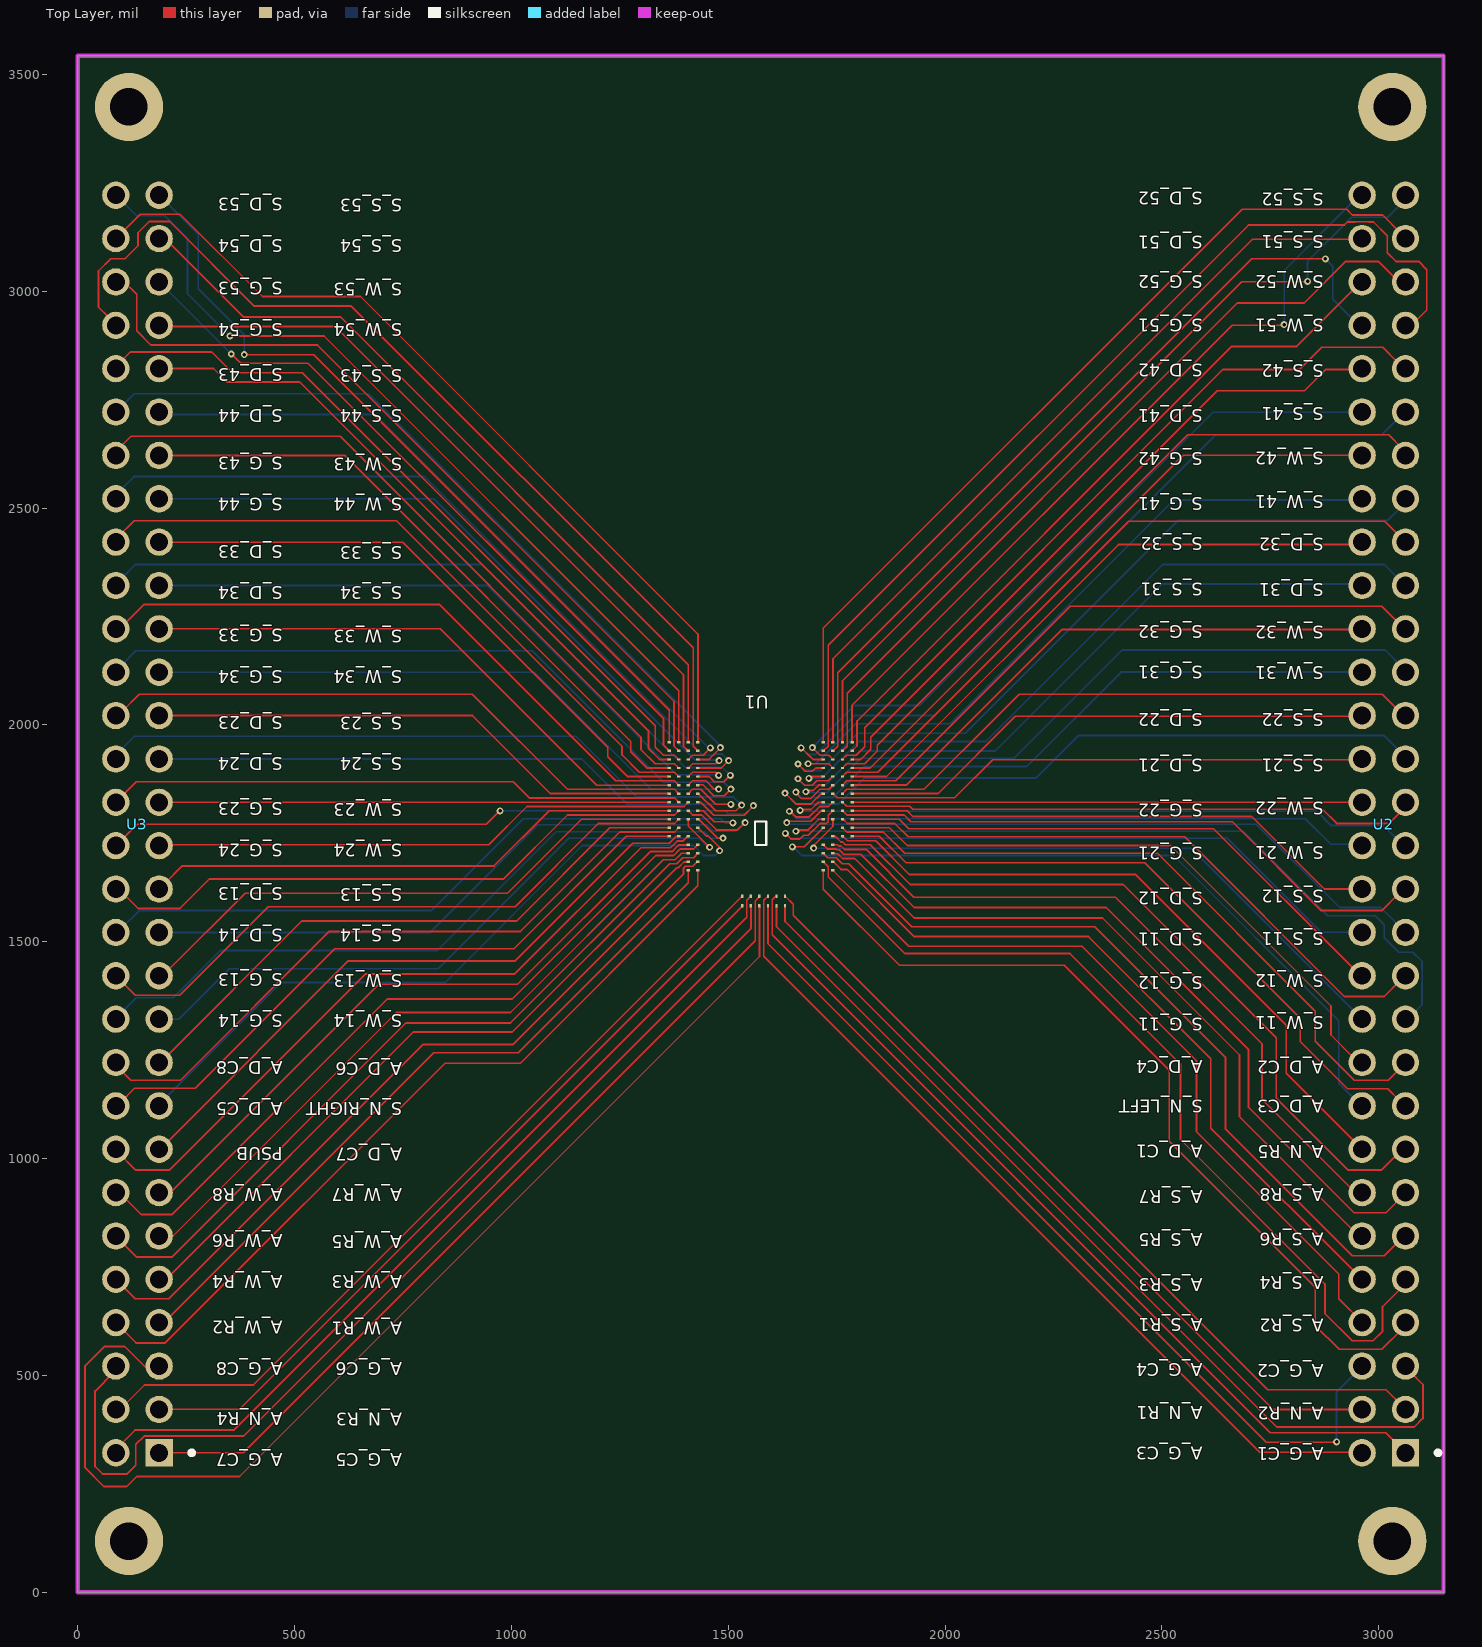
[diagram p0: Top Layer view]
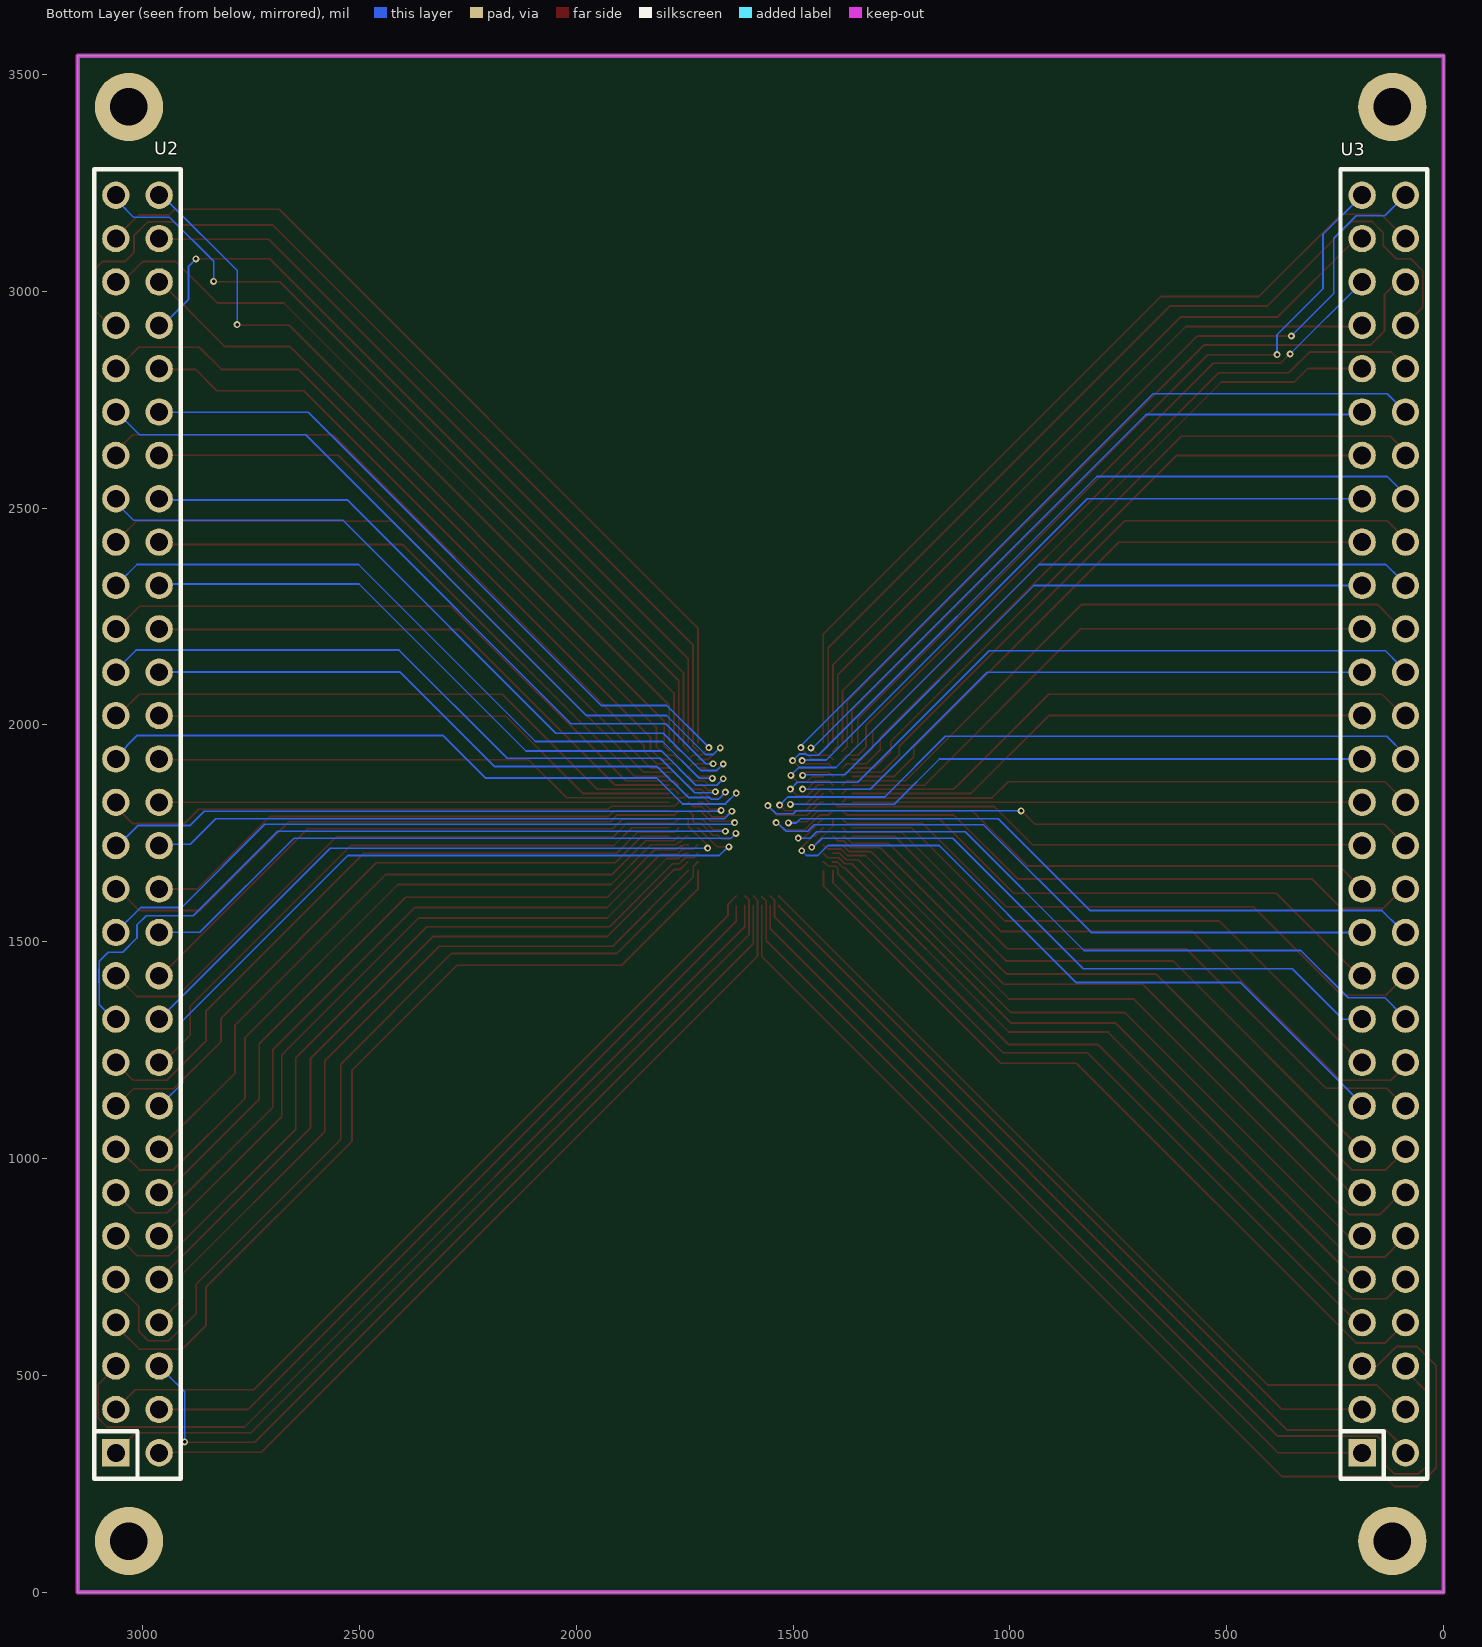
[diagram p1: Bottom Layer view, seen from below]
# Altium PCB MISC82787.pcbdoc
Units mil, origin at the board's own origin, x right, y up, seen from the top; angles counter-clockwise.
Board outline 3149.61 x 3543.31 mil, 2 copper layers (Top Layer, Bottom Layer); 3 components, 120 nets, 244 pads, 40 vias.

## Layer stack, top to bottom (the 12.6 mil dielectric is the usual default, probably not edited)
Top Layer: signal copper 1.4
Dielectric: dielectric 12.6, FR-4, Dk 4.8
Bottom Layer: signal copper 1.4

## Board outline
0,0 3149.61,0 3149.61,3543.31 0,3543.31

## Design rules (kind name [scope] priority, off if disabled: settings)
Clearance [All] p1: gap=5
MinimumSolderMaskSliver [All] p1: minsoldermaskwidth=0
PolygonConnect [All] p1: connectstyle=Relief reliefconductorwidth=10 reliefentries=4 polygonreliefangle="90 Angle"
RoutingVias [All] p1: holewidth=8 width=16 viastyle="Through Hole" minholewidth=8 minwidth=16 maxholewidth=8 maxwidth=16
SilkToSilkClearance [All] p1: silktosilkclearance=0
SilkscreenOverComponentPads [IsPad] p1: minsilkscreentomaskgap=0
SolderMaskExpansion [All] p1: expansion=4
Width [All] p1: maxlimit=4 minlimit=4 preferedwidth=4
25 further rules are at their usual default settings.

## Components (designator, comment, footprint, x,y, rotation, side; value= is the part's Value field where it differs from the comment)
U1 "" XP 1574.8,1771.65 r180 top locked
U2 "P125-1230A0BS116A1" HDR-TH_60P-P2.54-V-M-R2-C30-S2.54-1 3011.81,1771.65 r90 top locked
U3 "P125-1230A0BS116A1" HDR-TH_60P-P2.54-V-M-R2-C30-S2.54-1 137.8,1771.65 r90 top locked

## Footprints (in the part's own frame and the unit in brackets; to place one, negate y for a bottom-side part, rotate by r counter-clockwise, add the part's x,y. Pads: shape width x height; smd on the part's side, far side on the other; paste and mask are expansions set on the pad)
HDR-TH_60P-P2.54-V-M-R2-C30-S2.54-1 [mm]
  rect 1.6x1.6 hole 1.05: 1(-36.83,-1.27)
  round 1.6 hole 1.05: 2(-36.83,1.27) 3(-34.29,-1.27) 4(-34.29,1.27) 5(-31.75,-1.27) 6(-31.75,1.27) 7(-29.21,-1.27) 8(-29.21,1.27) 9(-26.67,-1.27) 10(-26.67,1.27) 11(-24.13,-1.27) 12(-24.13,1.27) 13(-21.59,-1.27) 14(-21.59,1.27) 15(-19.05,-1.27) 16(-19.05,1.27) 17(-16.51,-1.27) 18(-16.51,1.27) 19(-13.97,-1.27) 20(-13.97,1.27) 21(-11.43,-1.27) 22(-11.43,1.27) 23(-8.89,-1.27) 24(-8.89,1.27) 25(-6.35,-1.27) 26(-6.35,1.27) 27(-3.81,-1.27) 28(-3.81,1.27) 29(-1.27,-1.27) 30(-1.27,1.27) 31(1.27,-1.27) 32(1.27,1.27) 33(3.81,-1.27) 34(3.81,1.27) 35(6.35,-1.27) 36(6.35,1.27) 37(8.89,-1.27) 38(8.89,1.27) 39(11.43,-1.27) 40(11.43,1.27) 41(13.97,-1.27) 42(13.97,1.27) 43(16.51,-1.27) 44(16.51,1.27) 45(19.05,-1.27) 46(19.05,1.27) 47(21.59,-1.27) 48(21.59,1.27) 49(24.13,-1.27) 50(24.13,1.27) 51(26.67,-1.27) 52(26.67,1.27) 53(29.21,-1.27) 54(29.21,1.27) 55(31.75,-1.27) 56(31.75,1.27) 57(34.29,-1.27) 58(34.29,1.27) 59(36.83,-1.27) 60(36.83,1.27)
  silkscreen extent -36.96,-3.3 -36.7,-3.05
XP [mm]
  rect 0.14x0.2 smd: 1(-0.93,4.22) 2(-0.43,4.22) 3(-1.43,4.22) 4(-1.43,4.78) 5(-0.93,4.78) 6(-0.43,4.78) 115(0.07,4.78) 116(0.57,4.78) 117(1.07,4.78) 118(1.07,4.22) 119(0.07,4.22) 120(0.57,4.22)
  rect 0.2x0.14 smd: 7(-3.675,2.72) 8(-4.235,2.72) 9(-3.675,2.22) 10(-4.235,2.22) 11(-3.675,1.72) 12(-4.235,1.72) 13(-3.675,1.22) 14(-4.235,1.22) 15(-4.235,0.72) 16(-4.795,0.72) 17(-5.355,0.72) 18(-3.675,0.22) 19(-4.795,0.22) 20(-5.355,0.22) 21(-3.675,-0.28) 22(-4.235,-0.28) 23(-4.795,-0.28) 24(-5.355,-0.28) 25(-3.675,-0.78) 26(-4.235,-0.78) 27(-4.795,-0.78) 28(-5.355,-0.78) 29(-3.675,-1.28) 30(-4.235,-1.28) 31(-4.795,-1.28) 32(-5.355,-1.28) 33(-3.675,-1.78) 34(-4.235,-1.78) 35(-4.795,-1.78) 36(-5.355,-1.78) 37(-3.675,-2.28) 38(-4.235,-2.28) 39(-4.795,-2.28) 40(-5.355,-2.28) 41(-3.675,-2.78) 42(-4.235,-2.78) 43(-4.795,-2.78) 44(-5.355,-2.78) 45(-3.675,-3.28) 46(-4.235,-3.28) 47(-4.795,-3.28) 48(-5.355,-3.28) 49(-3.675,-3.78) 50(-4.235,-3.78) 51(-4.795,-3.78) 52(-5.355,-3.78) 53(-3.675,-4.28) 54(-4.235,-4.28) 55(-4.795,-4.28) 56(-5.355,-4.28) 57(-3.675,-4.78) 58(-4.235,-4.78) 59(-4.795,-4.78) 60(-5.355,-4.78) 61(5.355,-4.78) 62(4.795,-4.78) 63(4.235,-4.78) 64(3.675,-4.78) 65(5.355,-4.28) 66(4.795,-4.28) 67(4.235,-4.28) 68(3.675,-4.28) 69(5.355,-3.78) 70(4.795,-3.78) 71(4.235,-3.78) 72(3.675,-3.78) 73(5.355,-3.28) 74(4.795,-3.28) 75(4.235,-3.28) 76(3.675,-3.28) 77(5.355,-2.78) 78(4.795,-2.78) 79(4.235,-2.78) 80(3.675,-2.78) 81(5.355,-2.28) 82(4.795,-2.28) 83(4.235,-2.28) 84(3.675,-2.28) 85(5.355,-1.78) 86(4.795,-1.78) 87(4.235,-1.78) 88(3.675,-1.78) 89(5.355,-1.28) 90(4.795,-1.28) 91(4.235,-1.28) 92(3.675,-1.28) 93(5.355,-0.78) 94(4.795,-0.78) 95(4.235,-0.78) 96(3.675,-0.78) 97(5.355,-0.28) 98(4.795,-0.28) 99(4.235,-0.28) 100(3.675,-0.28) 101(5.355,0.22) 102(4.795,0.22) 103(3.675,0.22) 104(5.355,0.72) 105(4.795,0.72) 106(4.235,0.72) 107(4.235,1.22) 108(3.675,1.22) 109(4.235,1.72) 110(3.675,1.72) 111(4.235,2.22) 112(3.675,2.22) 113(4.235,2.72) 114(3.675,2.72)
  silkscreen extent -0.32,-0.14 0.33,1.23

## Part data
U1: library part Chip3Array

## Free pads (board coordinates)
  round 157.48 hole 86.61: 0(118.11,118.11) 0(118.11,3425.2) 0(3031.5,118.11) 0(3031.5,3425.2)

## Via types
v1: diameter 16, hole 8, Top Layer to Bottom Layer, 40 vias

## Nets (pads, with @x,y where several pads share a name; then routed paths per layer and width w, separated by ;. In a path a pad name is that pad's centre, name@x,y a point inside that pad or via, vN(x,y) a via of type N, cw(c..) or ccw(c..) an arc to the next point about the centre after c; other vN are vias at no path point)
A_D_C1: U1.16 U2.16 | length 1547.7
  Top Layer w4: U1.16 U1.16@1765.44,1741.44 ; U1.16@1766,1742 1775,1733 1840,1733 1918,1655 2440,1655 2787,1308 2787,1197 U2.16@2952,1032
A_D_C2: U1.19 U2.19 | length 1573.8
  Top Layer w4: U1.19 1773.34,1753.24 1857.76,1753.24 1907,1704 2490,1704 2854,1340 2854,1271 2944,1181 3022,1181 U2.19@3046,1205
A_D_C3: U1.17 U2.17 | length 1546.4
  Top Layer w4: U1.17 1848.69,1743.31 1910,1682 2461,1682 2819,1324 2819,1270 2928,1161 3021,1161 U2.17@3048,1134
A_D_C4: U1.20 U2.20 | length 1415.1
  Top Layer w4: U1.20 1872.01,1762.99 1913,1722 2520,1722 2890,1352 2890,1285 U2.20@2942,1233
A_D_C5: U1.104 U3.18 | length 1520.4
  Top Layer w4: U3.18@98,1129 131,1162 271,1162 593,1484 1006,1484 1265.31,1743.31 U1.104
A_D_C6: U1.101 U3.19 | length 1378.7
  Top Layer w4: U3.19@204,1235 517,1548 1012,1548 1226.99,1762.99 U1.101
A_D_C7: U1.105 U3.15 | length 1473.6
  Top Layer w4: U3.15@205,1037 624,1456 1009,1456 1280,1727 1364,1727 1364.26,1727 1380.57,1743.31 U1.105
A_D_C8: U1.102 U3.20 | length 1546.1
  Top Layer w4: U3.20@93,1210 122,1181 237,1181 580,1524 1021,1524 1250.06,1753.06 1376.09,1753.06 U1.102
A_G_C1: U1.1 U2.1 | length 2016
  Top Layer w4: U1.1@1610,1605 1601.66,1596.66 1601.66,1516.34 2750,368 3016,368 U2.1@3039,345 ; U1.1@1610.45,1604.55 U1.1
A_G_C2: U1.5 U2.5 | length 2143.2
  Top Layer w4: U1.5 1611.42,1534.58 2765,381 3082,381 3102,401 3102,479 U2.5@3074,507
A_G_C3: U1.2 U2.2 | length 1978.4
  Top Layer w4: U1.2 1581.98,1595.76 1581.98,1467.02 2726,323 U2.2@2944,323
A_G_C4: U1.6 U2.6 | length 2050.9
  Top Layer w4: U1.6 1591.73,1495.27 2741,346 2903,346 v1(2903,347)
  Bottom Layer w4: v1(2903,347) 2903,462 U2.6@2945,504
A_G_C5: U1.119 U3.1 | length 1969.3
  Top Layer w4: U3.1 381.65,321.65 1562.12,1502.12 1562.12,1594.12 U1.119@1572,1604
A_G_C6: U1.115 U3.5 | length 2634.6
  Top Layer w4: U3.5@182,520 155,520 108,567 62,567 17,522 17,287 60,244 113,244 136,267 373,267 1572.05,1466.05 U1.115
A_G_C7: U1.120 U3.2 | length 1995.8
  Top Layer w4: U3.2@102,344 132,374 360,374 1542.61,1556.61 1542.61,1595.76 U1.120
A_G_C8: U1.116 U3.6 | length 2356.3
  Top Layer w4: U3.6@83,507 40,464 40,290 57,273 114,273 134,293 134,341 153.15,360.15 382.15,360.15 1552.36,1530.36 U1.116
A_N_R1: U1.4 U2.4 | length 1832.9
  Top Layer w4: U1.4@1631,1583 1631,1547 2756.35,421.65 U2.4
A_N_R2: U1.3 U2.3 | length 1924.8
  Top Layer w4: U1.3 1649.81,1586.81 1649.81,1561.19 2744,467 3017,467 U2.3@3054,430
A_N_R3: U1.117 U3.3 | length 1819.8
  Top Layer w4: U3.3@195,422 373,422 1532.68,1581.68 U1.117
A_N_R4: U1.118 U3.4 | length 1909.3
  Top Layer w4: U3.4@109,433 154,478 405.17,478 U1.118
A_N_R5: U1.15 U2.15 | length 1715.6
  Top Layer w4: U1.15 1746.69,1743.31 1759.99,1730.01 1763.9,1730.01 1769.91,1724 1828,1724 1920,1632 2411,1632 2764,1279 2764,1139 2929,974 3007,974 U2.15@3042,1009
A_S_R1: U1.8 U2.8 | length 1784.2
  Top Layer w4: U1.8 1916.1,1490 2316,1490 2580,1226 2580,1062 2908,734 2908,677 U2.8@2964,621
A_S_R2: U1.7 U2.7 | length 1985.6
  Top Layer w4: U1.7 1719.49,1621.51 1895,1446 2275,1446 2517,1204 2517,1040 2854,703 2854,615 2908.85,560.15 3007.15,560.15 U2.7@3055,608
A_S_R3: U1.10 U2.10 | length 1710.9
  Top Layer w4: U1.10@1743,1684 1760,1667 1774,1667 1929,1512 2331,1512 2613,1230 2613,1070.46 U2.10
A_S_R4: U1.9 U2.9 | length 2032.3
  Top Layer w4: U1.9 1730.43,1673.32 1730.43,1649.57 1907,1473 2288,1473 2543,1218 2543,1044 2876,711 2876,643 2939,580 2987,580 3009,602 3009,659 U2.9@3054,704
A_S_R5: U1.12 U2.12 | length 1647.9
  Top Layer w4: U1.12 U1.12@1743.06,1703.94 ; U1.12@1742,1704 1746,1704 1746.99,1703.01 1752.72,1703.01 1763.73,1692 1792,1692 1929,1555 2363,1555 2679,1239 2679,1097 U2.12@2944,832
A_S_R6: U1.11 U2.11 | length 1817
  Top Layer w4: U1.11 1729.42,1694.01 1748.99,1694.01 1763,1680 1778,1680 1923,1535 2345,1535 2647,1233 2647,1068 2939,776 3013,776 U2.11@3043,806
A_S_R7: U1.14 U2.14 | length 1595.4
  Top Layer w4: U1.14 U1.14@1742.08,1723.08 ; U1.14@1743,1724 1752,1724 1754.99,1721.01 1760.18,1721.01 1768.18,1713 1818,1713 1928,1603 2393,1603 2731,1265 2731,1137 U2.14@2935,933
A_S_R8: U1.13 U2.13 | length 1773.6
  Top Layer w4: U1.13 1729.24,1713.87 1748.86,1713.87 1749.73,1713 1750.72,1712.01 1756.45,1712.01 1766.46,1702 1806,1702 1929,1579 2372,1579 2700,1251 2700,1118 2943,875 3017,875 U2.13@3050,908
A_W_R1: U1.113 U3.7 | length 1642.1
  Top Layer w4: U3.7@210,633 821,1244 1016,1244 1408.07,1636.07 U1.113
A_W_R2: U1.114 U3.8 | length 1833.1
  Top Layer w4: U3.8 134.45,575 202,575 847,1220 1021,1220 1430,1629 U1.114@1430,1664
A_W_R3: U1.111 U3.9 | length 1592.2
  Top Layer w4: U3.9@212,730 774,1292 1002,1292 1381,1671 1383,1671 1385,1671 1398,1684 1408.07,1684 U1.111@1409,1684
A_W_R4: U1.112 U3.10 | length 1785.2
  Top Layer w4: U3.10 132.45,677 210,677 796,1263 1003,1263 1397.13,1657.13 1397.13,1670.22 1401.23,1674.32 1415.1,1674.32 1418.32,1674.32 U1.112@1429,1685 ; U1.112@1429.93,1684.07 U1.112
A_W_R5: U1.109 U3.11 | length 1585.8
  Top Layer w4: U3.11 219.65,821.65 735,1337 998,1337 1350,1689 1374.27,1689 1377.27,1689 1390.22,1701.95 ; 1390.17,1702 1392.11,1703.94 U1.109 U1.109@1408,1703.94
A_W_R6: U1.110 U3.12 | length 1737.7
  Top Layer w4: U3.12@95,814 136,773 217,773 757,1313 998,1313 1365,1680 1381,1680 1395.01,1694.01 1420.19,1694.01 U1.110
A_W_R7: U1.107 U3.13 | length 1554.1
  Top Layer w4: U3.13 213.65,921.65 694,1402 1014,1402 1320,1708 1370.72,1708 1380.72,1718 1385.58,1722.87 1385.72,1723 1387.73,1723 1403,1723 U1.107@1408,1723 ; U1.107@1408,1723.62 U1.107 ; U1.107@1408.07,1723 U1.107@1410,1723
A_W_R8: U1.108 U3.14 | length 1689.4
  Top Layer w4: U3.14@110,908 147,871 217,871 714,1368 1002,1368 1333,1699 1374.45,1699 1388.45,1713 1389.31,1713.87 ; 1389.45,1714 1389.31,1713.87 ; U1.108@1428.75,1722.25 U1.108 ; U1.108@1429,1723 1420,1714 1415.04,1714 1415.04,1713.87 1407,1713.87 1389.31,1713.87
PSUB: U1.106 U3.16 | length 1648.6
  Top Layer w4: U3.16@94,1013 133,974 212,974 664,1426 1008,1426 1299,1717 1366.99,1717 1381.99,1732 1382.62,1732.62 1396.62,1732.62 U1.106@1407,1743 ; U1.106@1407.5,1742.5 U1.106@1408,1743 ; U1.106@1407.88,1743.12 U1.106
S_D_11: U1.26 U2.26 | length 1568.8
  Top Layer w4: v1(1632,1750) 1645,1737 1665,1737 1674,1746 1685,1746 1711.92,1772.92 1726.32,1772.92 1730.6,1777.2 1730.6,1791.43 U1.26
  Bottom Layer w4: v1(1632,1750) 1643,1739 2651,1739 2868,1522 U2.26@2956,1522
S_D_12: U1.28 U2.28 | length 1251
  Top Layer w4: U1.28 1912.64,1802.36 1926,1789 2707,1789 2874.35,1621.65 U2.28
S_D_13: U1.94 U3.28 | length 1392.7
  Top Layer w4: U3.28@102,1614 139,1577 236,1577 304,1645 982,1645 1129.43,1792.43 1376.09,1792.43 U1.94
S_D_14: U1.96 U3.26 | length 1610.2
  Top Layer w4: U1.96 1442.64,1802.36 1468,1777 1508,1777 v1(1511,1774)
  Bottom Layer w4: U3.26@102,1532 142,1572 815,1572 1027,1784 1483,1784 1493,1774 v1(1511,1774)
S_D_21: U1.34 U2.34 | length 1244
  Top Layer w4: U1.34 1751.29,1831.98 2021.98,1831.98 2110,1920 U2.34@2945,1920
S_D_22: U1.36 U2.36 | length 1238.2
  Top Layer w4: U1.36 1983.73,1841.73 2162,2020 U2.36@2950,2020
S_D_23: U1.86 U3.36 | length 1395.6
  Top Layer w4: U3.36@102,2031 142,2071 910,2071 1129.34,1851.66 1376.09,1851.66 U1.86
S_D_24: U1.88 U3.34 | length 1646.6
  Top Layer w4: U1.88 1431.27,1841.73 1471,1802 1518,1802 v1(1531,1815)
  Bottom Layer w4: U3.34@90,1933 131,1974 1149,1974 1289,1834 1512,1834 v1(1531,1815)
S_D_31: U1.41 U2.41 | length 1625.8
  Top Layer w4: v1(1686,1877) 1690.1,1881.1 U1.41
  Bottom Layer w4: v1(1686,1877) 1716,1877 1801,1962 2094,1962 2502,2370 3013,2370 U2.41@3055,2328
S_D_32: U1.43 U2.43 | length 1543.8
  Top Layer w4: U1.43 1773.48,1891 1845,1891 2424,2470 3014,2470 U2.43@3049,2435
S_D_33: U1.78 U3.44 | length 1564.4
  Top Layer w4: U3.44@93,2434 130,2471 735,2471 1255,1951 1255,1931 1295.14,1890.86 1376.27,1890.86 U1.78
S_D_34: U1.80 U3.42 | length 1707.5
  Top Layer w4: U1.80 1455.9,1881.1 1468,1869 1490,1869 v1(1505,1884)
  Bottom Layer w4: U3.42@99,2336 133,2370 933,2370 1401,1902 1487,1902 v1(1505,1884)
S_D_41: U1.50 U2.50 | length 1631.1
  Top Layer w4: v1(1694,1948) 1711.77,1930.23 1731.78,1930.23 U1.50
  Bottom Layer w4: v1(1694,1948) 1705,1959 1791,2045 1942,2045 2618,2721 U2.50@2946,2721
S_D_42: U1.52 U2.52 | length 1561.4
  Top Layer w4: U1.52 1805.47,1920.47 1829,1944 1829,1972 2628,2771 2829,2771 2878,2820 U2.52@2958,2820
S_D_43: U1.70 U3.52 | length 1720.4
  Top Layer w4: U3.52@96,2833 96,2835 121.15,2860.15 308.85,2860.15 357,2812 518,2812 1332,1998 1332,1949 1350.77,1930.23 1376.27,1930.23 U1.70
S_D_44: U1.72 U3.50 | length 1814.8
  Top Layer w4: U1.72 1455.47,1920.47 1482,1947 v1(1482,1948)
  Bottom Layer w4: U3.50 130.14,2764 670,2764 v1@1484,1950
S_D_51: U1.58 U2.58 | length 1810.9
  Top Layer w4: U1.58 1741.54,2152.54 2709,3120 U2.58@2959,3120
S_D_52: U1.60 U2.60 | length 1800.7
  Top Layer w4: U1.60 1785.63,2045.63 2662,2922 v1@2781,2922 ; v1@2782,2922 v1@2781,2922 ; v1(2782,2923) v1@2781,2922
  Bottom Layer w4: v1(2782,2923) 2782,3048 U2.60@2944,3210
S_D_53: U1.62 U3.60 | length 1965.1
  Top Layer w4: v1(351,2897) 568,2897 1386.02,2078.98 U1.62
  Bottom Layer w4: U3.60 135.45,3174 201,3174 253,3122 253,2995 v1(351,2897)
S_D_54: U1.64 U3.58 | length 2016.7
  Top Layer w4: U3.58 144.14,3178 236,3178 426,2988 652,2988 1430.12,2209.88 U1.64
S_G_11: U1.22 U2.22 | length 1509.7
  Top Layer w4: v1@1696,1716 v1(1697,1716) ; v1@1696,1721 1741.54,1766.54 U1.22
  Bottom Layer w4: v1(1697,1716) 2567.46,1716 U2.22
S_G_12: U1.24 U2.24 | length 1306.2
  Top Layer w4: U1.24 1894.32,1782.68 1916,1761 2619,1761 U2.24@2947,1433
S_G_13: U1.98 U3.24 | length 1473.4
  Top Layer w4: U3.24@96,1414 133,1377 235,1377 439,1581 1009,1581 1200.75,1772.75 1376.09,1772.75 U1.98
S_G_14: U1.100 U3.22 | length 1649
  Top Layer w4: U1.100 1432.32,1782.68 1476,1739 v1(1488,1739)
  Bottom Layer w4: U3.22@96,1332 135,1371 220,1371 329,1480 829,1480 1103,1754 1445,1754 1460,1739 v1(1488,1739)
S_G_21: U1.30 U2.30 | length 1459.8
  Top Layer w4: v1(1641,1801) v1@1644,1798 ; v1@1645,1799 1656,1788 1687,1788 1711.12,1812.12 1726.44,1812.12 1731.12,1812.12 U1.30@1741,1822 ; U1.30@1741.24,1821.76 U1.30
  Bottom Layer w4: v1@1640,1801 v1(1641,1801) 1658,1784 2831,1784 2890,1725 U2.30@2949,1725
S_G_22: U1.32 U2.32 | length 1158.3
  Top Layer w4: U1.32 U2.32@2943.95,1822.05
S_G_23: U1.90 U3.32 | length 1312.9
  Top Layer w4: U3.32@105,1839 135,1869 1004,1869 1041.2,1831.8 1376.27,1831.8 U1.90
S_G_24: U1.92 U3.30 | length 1655.9
  Top Layer w4: U3.30 137.14,1771 942,1771 v1@971,1800 ; U1.92 1436.95,1822.05 1467,1792 1537,1792 v1@1556,1811 ; v1@1555.5,1811.5 v1(1558,1814)
  Bottom Layer w4: v1(974,1802) 1409,1802 1493,1802 1500,1795 1539,1795 v1@1555,1811
S_G_31: U1.38 U2.38 | length 1514.5
  Top Layer w4: v1(1656,1845) v1@1659,1842 ; v1@1658,1841 1668,1831 1691,1831 1711.66,1851.66 1731.66,1851.66 1741.42,1861.42 U1.38
  Bottom Layer w4: v1(1656,1845) 1672,1829 1689,1829 1693,1833 1742,1833 1813,1904 2188,1904 2406,2122 U2.38@2938,2122
S_G_32: U1.40 U2.40 | length 1307.9
  Top Layer w4: U1.40 1910.42,1861.42 2269,2220 U2.40@2945,2220
S_G_33: U1.82 U3.40 | length 1462.1
  Top Layer w4: U3.40@113,2238 153,2278 834,2278 1240.83,1871.17 1376.27,1871.17 U1.82
S_G_34: U1.84 U3.38 | length 1641.8
  Top Layer w4: U1.84 U1.84@1431,1861.42 ; U1.84@1431,1862 1442,1862 1467,1837 1491,1837 v1(1506,1852)
  Bottom Layer w4: U3.38@102,2139 134,2171 1048,2171 1351,1868 1490,1868 v1(1506,1852)
S_G_41: U1.46 U2.46 | length 1580.7
  Top Layer w4: v1(1684.46,1910.54) 1731.78,1910.54 U1.46
  Bottom Layer w4: v1(1684.46,1910.54) 1701.54,1910.54 1794,2003 2012,2003 2528,2519 U2.46@2952,2519
S_G_42: U1.48 U2.48 | length 1459.1
  Top Layer w4: U1.48 1827.79,1900.79 2549,2622 U2.48@2946,2622
S_G_43: U1.74 U3.48 | length 1652.1
  Top Layer w4: U3.48@84,2627 123,2666 605,2666 1299,1972 1299,1943 1331.46,1910.54 1376.27,1910.54 U1.74
S_G_44: U1.76 U3.46 | length 1780.8
  Top Layer w4: U1.76 1483.79,1900.79 v1(1501,1918)
  Bottom Layer w4: U3.46@89,2532 130,2573 799,2573 1442,1930 1468,1930 1471,1933 1485.21,1933 1486.21,1932 1487,1932 v1(1501,1918)
S_G_51: U1.54 U2.54 | length 1869.8
  Top Layer w4: U1.54 1752.65,1951.27 1752.65,2120.65 2707,3075 v1(2877,3075)
  Bottom Layer w4: v1(2877,3075) 2894,3058 2894,2982 U2.54@2940,2936
S_G_52: U1.56 U2.56 | length 1637.8
  Top Layer w4: U1.56 1797,1951.53 1797,2009 2661,2873 2811,2873 U2.56@2947,3009
S_G_53: U1.66 U3.56 | length 1842.2
  Top Layer w4: U3.56@103,3026 136,2993 136,2909 169,2876 553,2876 1374.91,2054.09 1374.91,1951.27 U1.66
S_G_54: U1.68 U3.54 | length 2205.5
  Top Layer w4: U3.54@75,2941 70,2941 48,2963 48,3047 76,3075 109,3075 139,3105 139,3135 165,3161 212,3161 407,2966 631,2966 1419.18,2177.82 1419.18,1951.09 U1.68
S_N_LEFT: U1.18 U2.18 | length 1724.4
  Top Layer w4: v1(1648,1719) 1648,1717 1650,1719 1675.5,1719 U1.18
  Bottom Layer w4: v1(1648,1719) v1@1651,1719 ; v1@1651,1718 1670,1699 2527,1699 2908,1318 2908,1174 U2.18@2952,1130
S_N_RIGHT: U1.103 U3.17 | length 1616.7
  Top Layer w4: U1.103 1449.11,1744 1454,1744 1480,1718 v1(1480,1710)
  Bottom Layer w4: U3.17@197,1135 468,1406 847,1406 1163,1722 1420,1722 1443,1699 1469,1699 v1(1480,1710)
S_S_11: U1.25 U2.25 | length 1624
  Top Layer w4: v1(1635,1775) 1635,1774 v1@1635.5,1774.5 ; v1@1639,1778 1690,1778 1714.36,1802.36 U1.25
  Bottom Layer w4: v1(1635,1775) 1639,1771 2718,1771 2910,1579 3004.46,1579 U2.25
S_S_12: U1.27 U2.27 | length 1391.2
  Top Layer w4: U1.27 1773.34,1792.61 1905.39,1792.61 1921,1777 2663,1777 2868,1572 3007,1572 U2.27@3044,1609
S_S_13: U1.93 U3.27 | length 1233.7
  Top Layer w4: U3.27@200,1634 241,1675 960,1675 1087.36,1802.36 U1.93
S_S_14: U1.95 U3.25 | length 1620.5
  Top Layer w4: U1.95 1417.83,1792.61 1438.39,1792.61 1473,1758 1522,1758 v1(1539,1775)
  Bottom Layer w4: U3.25 812.65,1521.65 1061,1770 1451,1770 1466,1755 1516,1755 v1@1535,1774
S_S_21: U1.33 U2.33 | length 1634.8
  Top Layer w4: v1(1631,1843) 1656,1818 1691,1818 1714.73,1841.73 U1.33
  Bottom Layer w4: v1(1631,1843) 1656,1818 1755,1818 1815,1878 2210,1878 2308,1976 3012,1976 U2.33@3061,1927
S_S_22: U1.35 U2.35 | length 1393.1
  Top Layer w4: U1.35 1773.34,1851.49 1951.49,1851.49 2122.5,2022.5 ; 2124.5,2024.5 2122.5,2022.5 ; U2.35@3044,2035 3008,2071 2171,2071 2122.5,2022.5
S_S_23: U1.85 U3.35 | length 1250.6
  Top Layer w4: U3.35 910.35,2021.65 1090,1842 U1.85@1364,1842
S_S_24: U1.87 U3.33 | length 1473.1
  Top Layer w4: U1.87 1417.83,1851.49 1436.95,1851.49 1441.05,1847.39 1441.05,1846.95 1471,1817 v1(1506,1817)
  Bottom Layer w4: U3.33 1162.35,1921.65 1267,1817 v1@1501,1817
S_S_31: U1.42 U2.42 | length 1579.5
  Top Layer w4: v1(1661,1876) 1676,1861 1694,1861 1704.35,1871.35 1730.35,1871.35 1740.1,1881.1 U1.42
  Bottom Layer w4: v1(1661,1876) 1676,1861 1724,1861 1803,1940 2116,1940 2501,2325 U2.42@2947,2325
S_S_32: U1.44 U2.44 | length 1392.9
  Top Layer w4: U1.44 1865.1,1881.1 2400,2416 U2.44@2957,2416
S_S_33: U1.77 U3.43 | length 1412
  Top Layer w4: U3.43 749.35,2421.65 1222,1949 1222,1927 1268,1881 U1.77@1363,1881
S_S_34: U1.79 U3.41 | length 1546.9
  Top Layer w4: U1.79 1417.83,1890.86 1471.14,1890.86 v1(1478,1884)
  Bottom Layer w4: U3.41 944.35,2321.65 1381,1885 v1@1477,1885
S_S_41: U1.49 U2.49 | length 1770.9
  Top Layer w4: v1(1668,1947) v1@1669,1947 ; v1@1669,1948 v1@1669,1947 ; U1.49 1695.74,1920.47 1690.67,1925.54 1690.46,1925.54 v1@1669,1947
  Bottom Layer w4: v1@1672,1944 1684,1932 1702,1932 1792,2022 1977,2022 2624,2669 3007,2669 U2.49@3051,2713
S_S_42: U1.51 U2.51 | length 1713
  Top Layer w4: U1.51 1773.34,1930.23 1795.23,1930.23 1815,1950 1815,1994 2641,2820 2818,2820 2869,2871 3009,2871 U2.51@3043,2837
S_S_43: U1.69 U3.51 | length 1565.4
  Top Layer w4: U3.51@196,2822 313,2822 344,2791 512,2791 1316,1987 1316,1946 1341.53,1920.47 U1.69
S_S_44: U1.71 U3.49 | length 1634.4
  Top Layer w4: U1.71 1417.83,1930.23 1442.23,1930.23 v1(1459,1947)
  Bottom Layer w4: U3.49@205,2716 686,2716 1455,1947 v1(1459,1947)
S_S_51: U1.57 U2.57 | length 2016.5
  Top Layer w4: U1.57 1719.49,2223.49 2685,3189 2926,3189 2939,3176 3009,3176 U2.57@3050,3135
S_S_52: U1.59 U2.59 | length 1910.3
  Top Layer w4: U1.59 1763.58,2101.58 2684,3022 v1@2831,3022 ; v1@2835,3022 v1(2836,3023)
  Bottom Layer w4: v1(2836,3023) 2836,3069 2938,3171 3021,3171 U2.59@3053,3203
S_S_53: U1.61 U3.59 | length 1842.7
  Top Layer w4: v1(384,2854) 544,2854 1363.98,2034.02 U1.61
  Bottom Layer w4: U3.59 278,3131.45 278,3006 384,2900 v1(384,2854)
S_S_54: U1.63 U3.57 | length 1791.2
  Top Layer w4: U3.57@199,3112 211,3112 382,2941 606,2941 1408.07,2138.93 U1.63
S_W_11: U1.21 U2.21 | length 1790.9
  Top Layer w4: v1(1656,1755) 1659,1758 1684.27,1758 1708.19,1781.92 1708.92,1781.92 1709.68,1782.68 U1.21
  Bottom Layer w4: v1(1656,1755) 2688,1755 2882.85,1560.15 2991.85,1560.15 3013,1539 3013,1509 3046,1476 3079,1476 3100,1455 3100,1437.91 3100.31,1437.6 3100.31,1405.4 3100,1405.4 3100,1355 U2.21@3079,1334
S_W_12: U1.23 U2.23 | length 1470.5
  Top Layer w4: U1.23 U1.23@1764.13,1782.13 ; U1.23@1765,1783 1775.25,1772.75 1884.25,1772.75 1915,1742 2553,1742 2921,1374 3013,1374 U2.23@3050,1411
S_W_13: U1.97 U3.23 | length 1303.2
  Top Layer w4: U3.23@206,1432 386,1612 991,1612 1161.68,1782.68 U1.97
S_W_14: U1.99 U3.21 | length 1532.7
  Top Layer w4: U1.99 1408.07,1766.93 v1(1457,1718)
  Bottom Layer w4: U3.21 232.65,1321.65 349,1438 831,1438 1132,1739 1433,1739 v1@1454,1718
S_W_21: U1.29 U2.29 | length 1485.1
  Top Layer w4: v1(1666,1803) 1666,1802 1667,1801 v1@1671,1805 ; v1@1669,1805 v1@1671,1805 ; U1.29 1708.05,1822.05 1691,1805 v1@1671,1805
  Bottom Layer w4: v1(1666,1803) 1666,1802 1667,1801 2858,1801 2891,1768 3011,1768 U2.29@3053,1726
S_W_22: U1.31 U2.31 | length 1331.6
  Top Layer w4: U1.31 1773.34,1812.29 1918.71,1812.29 1925.5,1805.5 2870.5,1805.5 2903,1773 3024,1773 U2.31@3060,1809
S_W_23: U1.89 U3.31 | length 1175.9
  Top Layer w4: U3.31 U1.89@1363.65,1821.65
S_W_24: U1.91 U3.29 | length 1242.7
  Top Layer w4: U3.29@206,1724 948,1724 1036.12,1812.12 1398.14,1812.12 U1.91
S_W_31: U1.37 U2.37 | length 1572.1
  Top Layer w4: v1(1679,1846) 1681,1846 1684,1849 1696,1849 1708.42,1861.42 U1.37
  Bottom Layer w4: v1(1679,1846) 1679,1844 1727,1844 1806,1923 2159,1923 2409,2173 3015,2173 U2.37@3051,2137
S_W_32: U1.39 U2.39 | length 1485
  Top Layer w4: U1.39 1773.34,1871.17 1886.17,1871.17 2289,2274 3007,2274 U2.39@3057,2224
S_W_33: U1.81 U3.39 | length 1324.6
  Top Layer w4: U3.39 836.35,2221.65 1197,1861 U1.81@1363,1861
S_W_34: U1.83 U3.37 | length 1481.8
  Top Layer w4: U1.83 1417.83,1871.17 1448.83,1871.17 1468,1852 v1(1478,1852)
  Bottom Layer w4: U3.37 1052.35,2121.65 1322,1852 v1@1476,1852
S_W_41: U1.45 U2.45 | length 1720.6
  Top Layer w4: v1(1661,1910) 1678,1893 1694,1893 1701.79,1900.79 U1.45
  Bottom Layer w4: v1(1661,1910) 1676,1895 1713,1895 1799,1981 2047,1981 2538,2472 3021,2472 U2.45@3054,2505
S_W_42: U1.47 U2.47 | length 1630.5
  Top Layer w4: U1.47 1773.51,1910.72 1814.72,1910.72 1844,1940 1844,1953 2560,2669 3023,2669 U2.47@3055,2637
S_W_43: U1.73 U3.47 | length 1487.8
  Top Layer w4: U3.47 615.35,2621.65 1275,1962 1275,1938 1312,1901 U1.73@1363,1901
S_W_44: U1.75 U3.45 | length 1617.9
  Top Layer w4: U1.75 1417.83,1910.54 1471.54,1910.54 v1(1479,1918)
  Bottom Layer w4: U3.45 821.35,2521.65 1424,1919 v1@1478,1919
S_W_51: U1.53 U2.53 | length 2231.3
  Top Layer w4: U1.53 1730.6,1951.27 1730.6,2183.6 2700,3153 2921,3153 2928,3160 2945.72,3160 2945.72,3160.15 2977.76,3160.15 2977.91,3160 2988,3160 3020,3128 3020,3089 3040,3069 3092,3069 3111,3050 3111,2957 U2.53@3085,2931
S_W_52: U1.55 U2.55 | length 1828.5
  Top Layer w4: U1.55 1774.52,1951.09 1774.52,2073.52 2674,2973 2828,2973 2924,3069 2999,3069 U2.55@3037,3031
S_W_53: U1.65 U3.55 | length 1660
  Top Layer w4: v1@354,2856 354.28,2855.72 376,2834 531,2834 1351,2014 1351,1953.13 U1.65
  Bottom Layer w4: U3.55 v1(354,2855.45)
S_W_54: U1.67 U3.53 | length 1702
  Top Layer w4: U3.53@208,2919 594,2919 1396.96,2116.04 1396.96,1951.27 U1.67

## Keep-outs
Keep-Out Layer:
  the board outline again, w10

## Silkscreen, mask and mechanical layers (free items; w line width, h text height)
Top Overlay:
  text "S_D_52" at 2594,3240 h50 r180
  text "S_S_52" at 2873,3238 h50 r180
  text "S_D_53" at 473,3226 h50 r180
  text "S_S_53" at 748,3224 h50 r180
  text "S_S_51" at 2873,3140 h50 r180
  text "S_D_51" at 2594,3139 h50 r180
  text "S_D_54" at 473,3131 h50 r180
  text "S_S_54" at 748,3131 h50 r180
  text "S_G_52" at 2594,3048 h50 r180
  text "S_W_52" at 2873,3047 h50 r180
  text "S_G_53" at 473,3032 h50 r180
  text "S_W_53" at 748,3030 h50 r180
  text "S_G_51" at 2594,2947 h50 r180
  text "S_W_51" at 2873,2947 h50 r180
  text "S_G_54" at 473,2937 h50 r180
  text "S_W_54" at 748,2937 h50 r180
  text "S_D_42" at 2594,2843 h50 r180
  text "S_S_42" at 2873,2842 h50 r180
  text "S_D_43" at 473,2833 h50 r180
  text "S_S_43" at 748,2831 h50 r180
  text "S_S_41" at 2873,2743 h50 r180
  text "S_D_41" at 2594,2739 h50 r180
  text "S_D_44" at 473,2738 h50 r180
  text "S_S_44" at 748,2738 h50 r180
  text "S_W_42" at 2873,2641 h50 r180
  text "S_G_42" at 2594,2639 h50 r180
  text "S_G_43" at 473,2629 h50 r180
  text "S_W_43" at 748,2627 h50 r180
  text "S_W_41" at 2873,2540 h50 r180
  text "S_G_41" at 2594,2536 h50 r180
  text "S_G_44" at 473,2534 h50 r180
  text "S_W_44" at 748,2534 h50 r180
  text "S_S_32" at 2594,2443 h50 r180
  text "S_D_32" at 2873,2442 h50 r180
  text "S_D_33" at 473,2425 h50 r180
  text "S_S_33" at 748,2423 h50 r180
  text "S_S_31" at 2594,2338 h50 r180
  text "S_D_31" at 2873,2337 h50 r180
  text "S_D_34" at 473,2330 h50 r180
  text "S_S_34" at 748,2330 h50 r180
  text "S_G_32" at 2594,2240 h50 r180
  text "S_W_32" at 2873,2239 h50 r180
  text "S_G_33" at 473,2232 h50 r180
  text "S_W_33" at 748,2230 h50 r180
  text "S_G_31" at 2594,2147 h50 r180
  text "S_W_31" at 2873,2146 h50 r180
  text "S_G_34" at 473,2137 h50 r180
  text "S_W_34" at 748,2137 h50 r180
  text "S_D_22" at 2594,2037 h50 r180
  text "S_S_22" at 2873,2037 h50 r180
  text "S_D_23" at 473,2031 h50 r180
  text "S_S_23" at 748,2029 h50 r180
  text "S_D_24" at 473,1936 h50 r180
  text "S_S_24" at 748,1936 h50 r180
  text "S_D_21" at 2594,1933 h50 r180
  text "S_S_21" at 2873,1932 h50 r180
  text "S_W_22" at 2873,1833 h50 r180
  text "S_G_23" at 473,1832 h50 r180
  text "S_W_23" at 748,1830 h50 r180
  text "S_G_22" at 2594,1829 h50 r180
  text "S_G_24" at 473,1737 h50 r180
  text "S_W_24" at 748,1737 h50 r180
  text "S_W_21" at 2873,1731 h50 r180
  text "S_G_21" at 2594,1729 h50 r180
  text "S_D_13" at 473,1636 h50 r180
  text "S_S_13" at 748,1634 h50 r180
  text "S_S_12" at 2873,1630 h50 r180
  text "S_D_12" at 2594,1626 h50 r180
  text "S_D_14" at 473,1541 h50 r180
  text "S_S_14" at 748,1541 h50 r180
  text "S_S_11" at 2873,1532 h50 r180
  text "S_D_11" at 2594,1531 h50 r180
  text "S_G_13" at 473,1438 h50 r180
  text "S_W_13" at 748,1436 h50 r180
  text "S_W_12" at 2873,1435 h50 r180
  text "S_G_12" at 2594,1431 h50 r180
  text "S_G_14" at 473,1343 h50 r180
  text "S_W_14" at 748,1343 h50 r180
  text "S_W_11" at 2873,1339 h50 r180
  text "S_G_11" at 2594,1335 h50 r180
  text "A_D_C4" at 2594,1237 h50 r180
  text "A_D_C2" at 2873,1236 h50 r180
  text "A_D_C8" at 473,1235 h50 r180
  text "A_D_C6" at 748,1233 h50 r180
  text "S_N_LEFT" at 2594,1146 h50 r180
  text "A_D_C3" at 2873,1146 h50 r180
  text "A_D_C5" at 473,1140 h50 r180
  text "S_N_RIGHT" at 748,1140 h50 r180
  text "A_D_C1" at 2594,1042 h50 r180
  text "A_N_R5" at 2873,1041 h50 r180
  text "PSUB" at 473,1037 h50 r180
  text "A_D_C7" at 748,1035 h50 r180
  text "A_W_R8" at 473,942 h50 r180
  text "A_W_R7" at 748,942 h50 r180
  text "A_S_R8" at 2873,942 h50 r180
  text "A_S_R7" at 2594,938 h50 r180
  text "A_S_R6" at 2873,840 h50 r180
  text "A_S_R5" at 2594,838 h50 r180
  text "A_W_R6" at 473,836 h50 r180
  text "A_W_R5" at 748,834 h50 r180
  text "A_W_R4" at 473,741 h50 r180
  text "A_W_R3" at 748,741 h50 r180
  text "A_S_R4" at 2873,739 h50 r180
  text "A_S_R3" at 2594,735 h50 r180
  text "A_S_R1" at 2594,642 h50 r180
  text "A_S_R2" at 2873,641 h50 r180
  text "A_W_R2" at 473,636 h50 r180
  text "A_W_R1" at 748,634 h50 r180
  text "A_G_C8" at 473,541 h50 r180
  text "A_G_C6" at 748,541 h50 r180
  text "A_G_C4" at 2594,539 h50 r180
  text "A_G_C2" at 2873,536 h50 r180
  text "A_N_R1" at 2594,439 h50 r180
  text "A_N_R2" at 2873,438 h50 r180
  text "A_N_R4" at 473,426 h50 r180
  text "A_N_R3" at 748,424 h50 r180
  text "A_G_C3" at 2594,346 h50 r180
  text "A_G_C1" at 2873,345 h50 r180
  text "A_G_C7" at 473,331 h50 r180
  text "A_G_C5" at 748,331 h50 r180